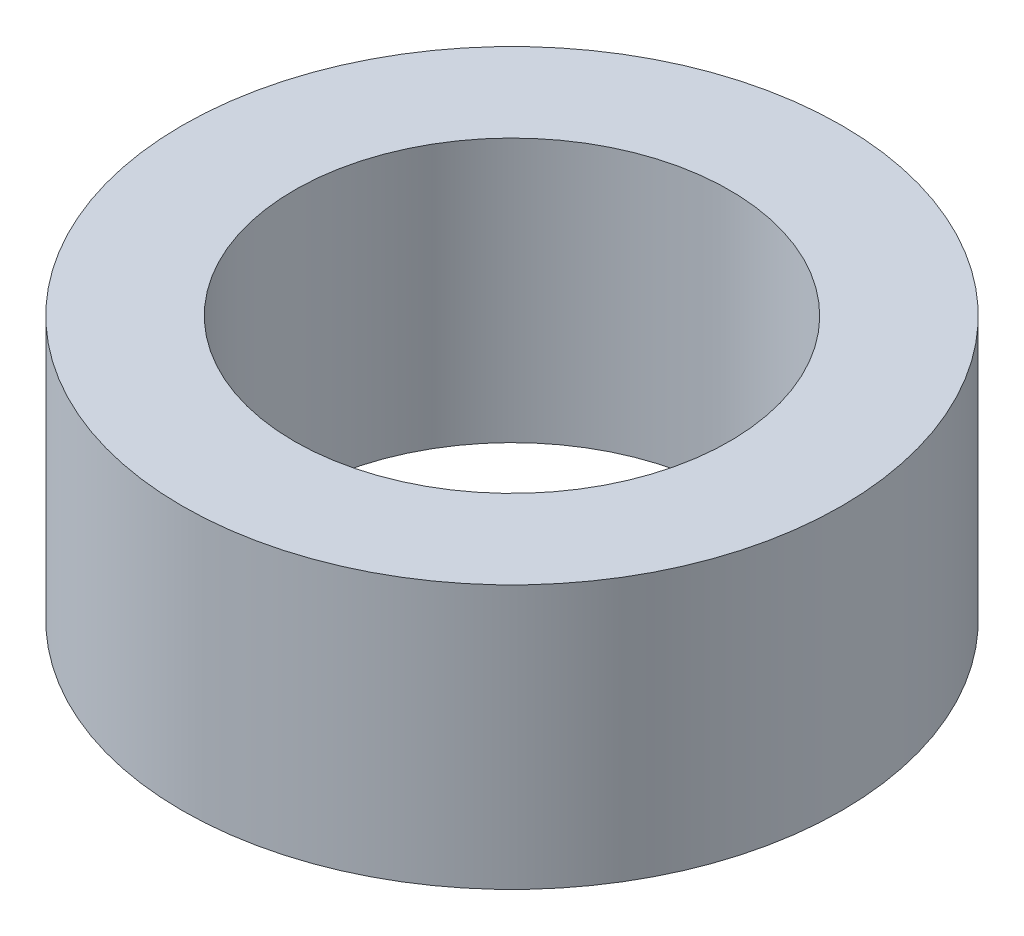
from build123d import *

# Parameters (mm, degrees)
SKETCH1_R           = 12.5
SKETCH1_R_2         = 8.25
BOSS_EXTRUDE1_DEPTH = 10


with BuildPart() as part:
    # Sketch1 → Boss-Extrude1 (new body)
    with BuildSketch(Plane(origin=(0, 0, 0), x_dir=(1, 0, 0), z_dir=(0, 1, 0))):
        with Locations(Location((0, 0, 0), (0, 0, 270))):
            Circle(SKETCH1_R)
        with Locations(Location((0, 0, 0), (0, 0, 270))):
            Circle(SKETCH1_R_2, mode=Mode.SUBTRACT)
    extrude(amount=BOSS_EXTRUDE1_DEPTH)


solid = part.part
